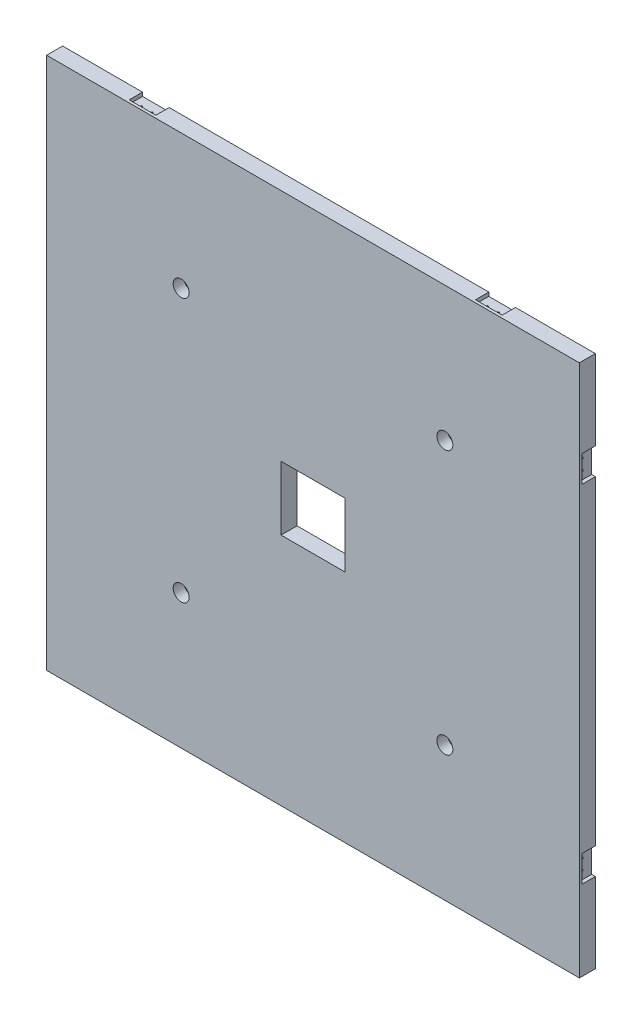
SolidWorks part; units mm, degrees
ref_plane "Front Plane" through (0, 0, 0) normal (0, 0, 1) x (1, 0, 0)
ref_plane "Top Plane" through (0, 0, 0) normal (0, 1, 0) x (1, 0, 0)
ref_plane "Right Plane" through (0, 0, 0) normal (1, 0, 0) x (0, 0, -1)
sketch "Sketch1" plane through (0, 0, 0) normal (0, 0, 1) x (1, 0, 0)
  line L1 (-500, -500) -> (500, -500)
  line L2 (-500, -500) -> (-500, 500)
  line L3 (-500, 500) -> (500, 500)
  line L4 (500, -500) -> (500, 500)
  line L5 (0, 500) -> (0, -500) construction
  line L6 (-500, 0) -> (500, 0) construction
  line L7 (-60, -60) -> (60, -60)
  line L8 (-60, -60) -> (-60, 60)
  line L9 (-60, 60) -> (60, 60)
  line L10 (60, -60) -> (60, 60)
  line L11 (0, 60) -> (0, -60) construction
  line L12 (-60, 0) -> (60, 0) construction
  point P0 (0, 0)
  point P4 (0, 0)
  dimension "D1" = 1000
  dimension "D2" = 1000
  dimension "D3" = 120
extrude "Boss-Extrude1" add sketch "Sketch1" along normal blind 30
sketch "Sketch2" plane through (0, 0, 30) normal (0, 0, 1) x (1, 0, 0)
  line L0 (0, 0) -> (-500, 500) construction
  line L1 (0, 0) -> (-247.4874, 247.4874) construction
  circle A0 centre (-247.4874, 247.4874) radius 15
  circle A1 centre (0, 0) radius 350 construction
  circle A2 centre (247.4874, 247.4874) radius 15
  circle A3 centre (247.4874, -247.4874) radius 15
  circle A4 centre (-247.4874, -247.4874) radius 15
  dimension "D1" = 30
  dimension "D2" = 700
  dimension "D3" = 4
extrude "Cut-Extrude1" cut sketch "Sketch2" against normal blind 20
sketch "Sketch3" plane through (0, 500, 0) normal (0, 1, 0) x (1, 0, 0)
  line L0 (0, 0) -> (0, 247.7781) construction
  line L1 (-350, 65) -> (-300, 65)
  line L2 (-350, 65) -> (-350, -25)
  line L3 (-350, -25) -> (-300, -25)
  line L4 (-300, 65) -> (-300, -25)
  line L5 (500, 0) -> (-500, 0) construction
  line L6 (300, 65) -> (300, -25)
  line L7 (350, -25) -> (300, -25)
  line L8 (350, 65) -> (350, -25)
  line L9 (350, 65) -> (300, 65)
  line L10 (500, -30) -> (-500, -30) construction
  dimension "D1" = 150
  dimension "D2" = 5
  dimension "D3" = 90
  dimension "D4" = 50
extrude "Cut-Extrude2" cut sketch "Sketch3" against normal blind 7
sketch "Sketch4" plane through (0, 0, 0) normal (0, 1, 0) x (1, 0, 0)
  line L0 (0, 0) -> (0, 211.2363) construction
pattern_circular "CirPattern1" count 4 over 360 about axis through (0, 0, 0) along (0, 0, 1) of "Cut-Extrude2"
hole_wizard "M4 Tapped Hole1" positions "Sketch5" profile "Sketch6" tap size "M4" standard "GB"
sketch "Sketch5" plane through (0, -493, 0) normal (0, -1, 0) x (-1, 0, 0)
  point P0 (-335, -17.5)
  point P6 (-315, -17.5)
  point P11 (315, -17.5)
  point P14 (335, -17.5)
sketch "Sketch6" plane through (335, -493, 17.5) normal (1, 0, 0) x (0, 0, -1)
  line L0 (0, 0) -> (0, 11.0914)
  line L1 (0, 11.0914) -> (1.65, 10.1)
  line L2 (1.65, 10.1) -> (1.65, 0)
  line L5 (1.65, 0) -> (0, 0)
  line L10 (0, 11.0914) -> (-1.65, 10.1) construction
  line L11 (0, -6.35) -> (0, 107.95) construction
  dimension "螺纹孔钻头直径" = 3.3
  dimension "螺纹孔钻头深度" = 10.1
  dimension "导头角度" = 118
cosmetic thread "Cosmetic thread 1" parameters "D1"=8, "D2"=4
cosmetic thread "Cosmetic thread 2" parameters "D1"=8, "D2"=4
cosmetic thread "Cosmetic thread 3" parameters "D1"=8, "D2"=4
cosmetic thread "Cosmetic thread 4" parameters "D1"=8, "D2"=4
pattern_circular "CirPattern2" count 4 every 90 about axis through (0, 0, 0) along (0, 0, -1) of "M4 Tapped Hole1"
cosmetic thread "Cosmetic thread 5" parameters "D1"=8, "D2"=4
cosmetic thread "Cosmetic thread 6" parameters "D1"=8, "D2"=4
cosmetic thread "Cosmetic thread 7" parameters "D1"=8, "D2"=4
cosmetic thread "Cosmetic thread 8" parameters "D1"=8, "D2"=4
cosmetic thread "Cosmetic thread 9" parameters "D1"=8, "D2"=4
cosmetic thread "Cosmetic thread 10" parameters "D1"=8, "D2"=4
cosmetic thread "Cosmetic thread 11" parameters "D1"=8, "D2"=4
cosmetic thread "Cosmetic thread 12" parameters "D1"=8, "D2"=4
cosmetic thread "Cosmetic thread 13" parameters "D1"=8, "D2"=4
cosmetic thread "Cosmetic thread 14" parameters "D1"=8, "D2"=4
cosmetic thread "Cosmetic thread 15" parameters "D1"=8, "D2"=4
cosmetic thread "Cosmetic thread 16" parameters "D1"=8, "D2"=4
